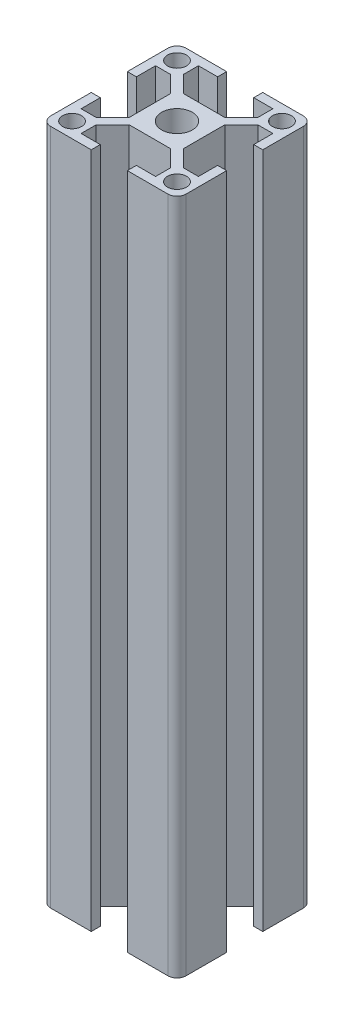
from build123d import *

# Parameters (mm, degrees)
SKETCH_1_R      = 2.1
SKETCH_1_R_2    = 3.4
EXTRUDE_1_DEPTH = 150


with BuildPart() as part:
    # 草图1 → 拉伸1 (new body)
    with BuildSketch(Plane(origin=(0, 0, 0), x_dir=(1, 0, 0), z_dir=(0, 1, 0))):
        with BuildLine():
            Line((6.75, -28), (11, -28))
            Line((11, -28), (11, -30))
            Line((11, -30), (2, -30))
            ThreePointArc((2, -30), (0.585786438, -29.414213562), (0, -28))
            Line((0, -28), (0, -19))
            Line((0, -19), (2, -19))
            Line((2, -19), (2, -23.25))
            Line((2, -23.25), (5.335785999, -23.25))
            Line((5.335785999, -23.25), (9, -19.585785999))
            Line((9, -19.585785999), (9, -10.414214001))
            Line((9, -10.414214001), (5.335785999, -6.75))
            Line((5.335785999, -6.75), (2, -6.75))
            Line((2, -6.75), (2, -11))
            Line((2, -11), (0, -11))
            Line((0, -11), (0, -2))
            ThreePointArc((0, -2), (0.585786438, -0.585786438), (2, 0))
            Line((2, 0), (11, 0))
            Line((11, 0), (11, -2))
            Line((11, -2), (6.75, -2))
            Line((6.75, -2), (6.75, -5.335785999))
            Line((6.75, -5.335785999), (10.414214001, -9))
            Line((10.414214001, -9), (19.585785999, -9))
            Line((19.585785999, -9), (23.25, -5.335785999))
            Line((23.25, -5.335785999), (23.25, -2))
            Line((23.25, -2), (19, -2))
            Line((19, -2), (19, 0))
            Line((19, 0), (28, 0))
            ThreePointArc((28, 0), (29.414213562, -0.585786438), (30, -2))
            Line((30, -2), (30, -11))
            Line((30, -11), (28, -11))
            Line((28, -11), (28, -6.75))
            Line((28, -6.75), (24.664214001, -6.75))
            Line((24.664214001, -6.75), (21, -10.414214001))
            Line((21, -10.414214001), (21, -19.585785999))
            Line((21, -19.585785999), (24.664214001, -23.25))
            Line((24.664214001, -23.25), (28, -23.25))
            Line((28, -23.25), (28, -19))
            Line((28, -19), (30, -19))
            Line((30, -19), (30, -28))
            ThreePointArc((30, -28), (29.414213562, -29.414213562), (28, -30))
            Line((28, -30), (19, -30))
            Line((19, -30), (19, -28))
            Line((19, -28), (23.25, -28))
            Line((23.25, -28), (23.25, -24.664214001))
            Line((23.25, -24.664214001), (19.585785999, -21))
            Line((19.585785999, -21), (10.414214001, -21))
            Line((10.414214001, -21), (6.75, -24.664214001))
            Line((6.75, -24.664214001), (6.75, -28))
        make_face()
        with Locations(Location((3.375, -26.625, 0), (0, 0, 270))):
            Circle(SKETCH_1_R, mode=Mode.SUBTRACT)
        with Locations(Location((26.625, -26.625, 0), (0, 0, 270))):
            Circle(SKETCH_1_R, mode=Mode.SUBTRACT)
        with Locations(Location((15, -15, 0), (0, 0, 270))):
            Circle(SKETCH_1_R_2, mode=Mode.SUBTRACT)
        with Locations(Location((3.375, -3.375, 0), (0, 0, 270))):
            Circle(SKETCH_1_R, mode=Mode.SUBTRACT)
        with Locations(Location((26.625, -3.375, 0), (0, 0, 270))):
            Circle(SKETCH_1_R, mode=Mode.SUBTRACT)
    extrude(amount=EXTRUDE_1_DEPTH)


solid = part.part
